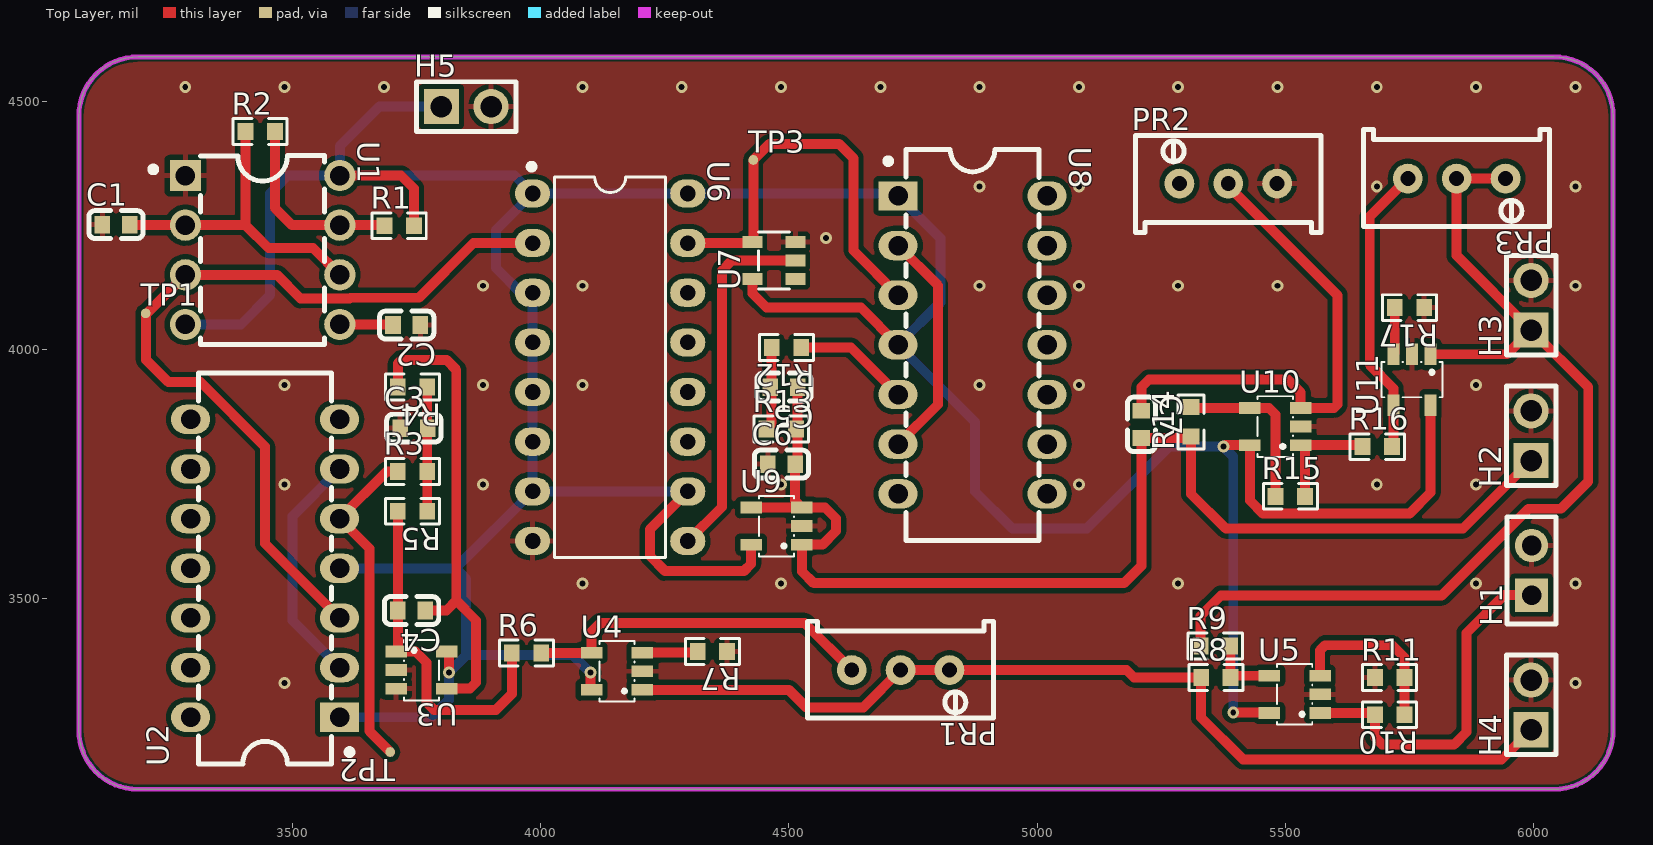
[diagram p0: Top Layer view]
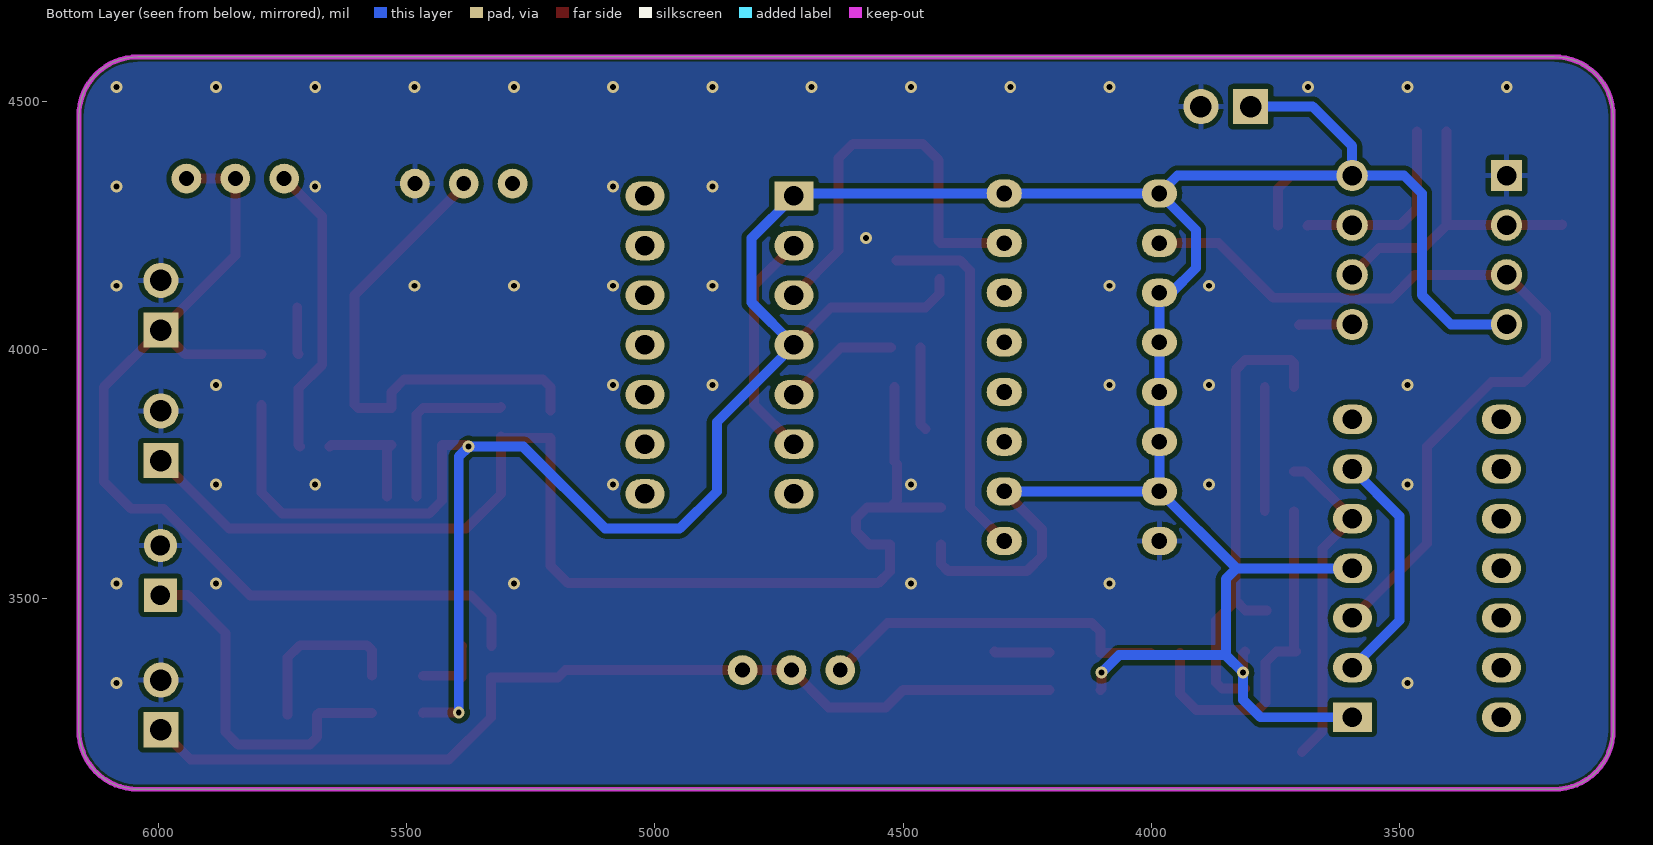
[diagram p1: Bottom Layer view, seen from below]
# Altium PCB MISC51901.pcbdoc
Units mil, origin at the board's own origin, x right, y up, seen from the top; angles counter-clockwise.
Board outline 3090 x 1475 mil, 2 copper layers (Top Layer, Bottom Layer), stack 62.206 mil thick; 46 components, 29 nets, 157 pads, 49 vias.

## Layer stack, top to bottom
Top Solder Mask Layer: solder mask 0.394, Dk 3.3
Top Layer: signal copper 1.379
Dielectric1: surface 59.449, FR4, Dk 4.5
Bottom Layer: signal copper 1.378
Bottom Solder Mask Layer: solder mask 0.394, Dk 3.3

## Board outline
3188.11,4590 ccw(c3188.11,4471.89) 3070,4471.89 3070,3233.11 ccw(c3188.11,3233.11) 3188.11,3115 6041.89,3115 ccw(c6041.89,3233.11) 6160,3233.11 6160,4471.89 ccw(c6041.89,4471.89) 6041.89,4590

## Design rules (kind name [scope] priority, off if disabled: settings)
BoardOutlineClearance copperThickness2oz_1 [All] p2 off: genericclearance=7.99 ignorepadtopadclearanceinfootprint=FALSE except(0: Arc-SplitContinuation Track-SplitContinuation SMDPad-SplitContinuation THPad-SplitContinuation Via-SplitContinuation Fill-SplitContinuation Region-SplitContinuation Poly-SplitContinuation Text-SplitContinuation Hole-SplitContinuation; 5.98: Arc-CutoutEdge Track-CutoutEdge SMDPad-CutoutEdge THPad-CutoutEdge Via-CutoutEdge Text-CutoutEdge; 6.9: Hole-OutlineEdge Hole-CutoutEdge; 10: Poly-OutlineEdge Poly-CutoutEdge; 11.81: Arc-OutlineEdge Track-OutlineEdge SMDPad-OutlineEdge THPad-OutlineEdge Via-OutlineEdge Fill-OutlineEdge Region-OutlineEdge Text-OutlineEdge Fill-CutoutEdge Region-CutoutEdge)
BoardOutlineClearance Plane_innerPlane_1 [All] p4 off: genericclearance=4.02 ignorepadtopadclearanceinfootprint=FALSE except(0: Arc-SplitContinuation Track-SplitContinuation SMDPad-SplitContinuation THPad-SplitContinuation Via-SplitContinuation Fill-SplitContinuation Region-SplitContinuation Poly-SplitContinuation Text-SplitContinuation Hole-SplitContinuation; 5.98: Arc-CutoutEdge Track-CutoutEdge SMDPad-CutoutEdge THPad-CutoutEdge Via-CutoutEdge Text-CutoutEdge; 6.9: Hole-OutlineEdge Hole-CutoutEdge; 10: Poly-OutlineEdge Poly-CutoutEdge; 11.81: Arc-OutlineEdge Track-OutlineEdge SMDPad-OutlineEdge THPad-OutlineEdge Via-OutlineEdge Fill-OutlineEdge Region-OutlineEdge Text-OutlineEdge Fill-CutoutEdge Region-CutoutEdge)
BoardOutlineClearance Copper_copperRegion_1 [All] p6 off: genericclearance=4.02 ignorepadtopadclearanceinfootprint=FALSE except(0: Arc-SplitContinuation Track-SplitContinuation SMDPad-SplitContinuation THPad-SplitContinuation Via-SplitContinuation Fill-SplitContinuation Region-SplitContinuation Poly-SplitContinuation Text-SplitContinuation Hole-SplitContinuation; 5.98: Arc-CutoutEdge Track-CutoutEdge SMDPad-CutoutEdge THPad-CutoutEdge Via-CutoutEdge Text-CutoutEdge; 6.9: Hole-OutlineEdge Hole-CutoutEdge; 10: Poly-OutlineEdge Poly-CutoutEdge; 11.81: Arc-OutlineEdge Track-OutlineEdge SMDPad-OutlineEdge THPad-OutlineEdge Via-OutlineEdge Fill-OutlineEdge Region-OutlineEdge Text-OutlineEdge Fill-CutoutEdge Region-CutoutEdge)
BoardOutlineClearance copperThickness1oz_1 [All] p8: genericclearance=4.02 ignorepadtopadclearanceinfootprint=FALSE except(0: Arc-SplitContinuation Track-SplitContinuation SMDPad-SplitContinuation THPad-SplitContinuation Via-SplitContinuation Fill-SplitContinuation Region-SplitContinuation Poly-SplitContinuation Text-SplitContinuation Hole-SplitContinuation; 5.98: Arc-CutoutEdge Track-CutoutEdge SMDPad-CutoutEdge THPad-CutoutEdge Via-CutoutEdge Text-CutoutEdge; 6.9: Hole-OutlineEdge Hole-CutoutEdge; 10: Poly-OutlineEdge Poly-CutoutEdge; 11.81: Arc-OutlineEdge Track-OutlineEdge SMDPad-OutlineEdge THPad-OutlineEdge Via-OutlineEdge Fill-OutlineEdge Region-OutlineEdge Text-OutlineEdge Fill-CutoutEdge Region-CutoutEdge)
Clearance copperThickness2oz [All] p1 off: gap=7.99 ignorepadtopadclearanceinfootprint=FALSE except(5.98: SMDPad-Track SMDPad-SMDPad THPad-Track SMDPad-THPad THPad-THPad Track-Via SMDPad-Via THPad-Via Via-Via Fill-SMDPad Region-SMDPad Fill-THPad Region-THPad Fill-Via Region-Via Fill-Fill Fill-Region Region-Region Arc-Track Arc-SMDPad Arc-THPad Arc-Via Fill-Arc Region-Arc Arc-Arc Text-Track SMDPad-Text Text-THPad Text-Via Fill-Text Region-Text Arc-Text Text-Text; 6.9: Hole-Track Hole-SMDPad Hole-THPad Hole-Via Fill-Hole Region-Hole Hole-Arc Hole-Text; 10: Poly-Track Poly-SMDPad Poly-THPad Poly-Via Poly-Fill Poly-Region Poly-Poly Poly-Arc Poly-Text Poly-Hole; 11.81: Fill-Track Region-Track)
Clearance Plane_innerPlane [All] p3 off: gap=4.02 ignorepadtopadclearanceinfootprint=FALSE except(5.98: SMDPad-Track SMDPad-SMDPad THPad-Track SMDPad-THPad THPad-THPad Track-Via SMDPad-Via THPad-Via Via-Via Fill-SMDPad Region-SMDPad Fill-THPad Region-THPad Fill-Via Region-Via Fill-Fill Fill-Region Region-Region Arc-Track Arc-SMDPad Arc-THPad Arc-Via Fill-Arc Region-Arc Arc-Arc Text-Track SMDPad-Text Text-THPad Text-Via Fill-Text Region-Text Arc-Text Text-Text; 6.9: Hole-Track Hole-SMDPad Hole-THPad Hole-Via Fill-Hole Region-Hole Hole-Arc Hole-Text; 10: Poly-Track Poly-SMDPad Poly-THPad Poly-Via Poly-Fill Poly-Region Poly-Poly Poly-Arc Poly-Text Poly-Hole; 11.81: Fill-Track Region-Track)
Clearance Copper_copperRegion [All] p5 off: gap=4.02 ignorepadtopadclearanceinfootprint=FALSE except(5.98: SMDPad-Track SMDPad-SMDPad THPad-Track SMDPad-THPad THPad-THPad Track-Via SMDPad-Via THPad-Via Via-Via Fill-SMDPad Region-SMDPad Fill-THPad Region-THPad Fill-Via Region-Via Fill-Fill Fill-Region Region-Region Arc-Track Arc-SMDPad Arc-THPad Arc-Via Fill-Arc Region-Arc Arc-Arc Text-Track SMDPad-Text Text-THPad Text-Via Fill-Text Region-Text Arc-Text Text-Text; 6.9: Hole-Track Hole-SMDPad Hole-THPad Hole-Via Fill-Hole Region-Hole Hole-Arc Hole-Text; 10: Poly-Track Poly-SMDPad Poly-THPad Poly-Via Poly-Fill Poly-Region Poly-Poly Poly-Arc Poly-Text Poly-Hole; 11.81: Fill-Track Region-Track)
Clearance copperThickness1oz [All] p7: gap=4.02 ignorepadtopadclearanceinfootprint=FALSE except(5.98: SMDPad-Track SMDPad-SMDPad THPad-Track SMDPad-THPad THPad-THPad Track-Via SMDPad-Via THPad-Via Via-Via Fill-SMDPad Region-SMDPad Fill-THPad Region-THPad Fill-Via Region-Via Fill-Fill Fill-Region Region-Region Arc-Track Arc-SMDPad Arc-THPad Arc-Via Fill-Arc Region-Arc Arc-Arc Text-Track SMDPad-Text Text-THPad Text-Via Fill-Text Region-Text Arc-Text Text-Text; 6.9: Hole-Track Hole-SMDPad Hole-THPad Hole-Via Fill-Hole Region-Hole Hole-Arc Hole-Text; 10: Poly-Track Poly-SMDPad Poly-THPad Poly-Via Poly-Fill Poly-Region Poly-Poly Poly-Arc Poly-Text Poly-Hole; 11.81: Fill-Track Region-Track)
DiffPairsRouting differentialPair [All] p1: maxlimit=6 minlimit=6 mostfreqgap=6 toplayer_minwidth=5 toplayer_prefwidth=10 toplayer_maxwidth=100 toplayer_mingap=6 toplayer_prefgap=6 toplayer_maxgap=6 bottomlayer_minwidth=5 bottomlayer_prefwidth=10 bottomlayer_maxwidth=100 bottomlayer_mingap=6 bottomlayer_prefgap=6 bottomlayer_maxgap=6 maxuncoupledlength=10
HoleToHoleClearance otherClearance [All] p1: gap=11.81 allowstackedmicrovias=TRUE
Length netLength [All] p1: minlimit=0 maxlimit=0
PasteMaskExpansion pasteMaskExpansion [All] p1: expansion=0
PlaneConnect innerPlane [All] p1: planeconnectstyle=Relief reliefexpansion=20 reliefentries=4 reliefconductorwidth=10 reliefairgap=10
PolygonConnect copperRegion [All] p1: connectstyle=Relief reliefconductorwidth=10 reliefentries=4 polygonreliefangle="90 Angle" airgapwidth=10 via.connectstyle=Relief via.reliefconductorwidth=10 via.reliefentries=4 via.polygonreliefangle="90 Angle" via.airgapwidth=10
RoutingVias viaSize [All] p1: holewidth=12.01 width=24.02 viastyle="Through Hole" minholewidth=11.81 minwidth=19.68 maxholewidth=248.03 maxwidth=393.7
SolderMaskExpansion solderMaskExpansion [IsVia] p1: expansion=-1000 istentingtop=TRUE
SolderMaskExpansion solderMaskExpansion [All] p2: expansion=2 istentingtop=FALSE
Width copperThickness2oz_2 [All] p1 off: maxlimit=100 minlimit=8 preferedwidth=10
Width copperThickness1oz_2 [All] p2: maxlimit=100 minlimit=5 preferedwidth=10

## Components (designator, comment, footprint, x,y, rotation, side; value= is the part's Value field where it differs from the comment)
C1 "5nF" C0603 3144.72,4252.4 r0 top
C2 "0.22uF" C0603 3730,4050 r180 top
C3 "5.1nF" C0603 3744.64,3842.36 r0 top
C4 "1nF" C0603 3740,3475 r180 top
C5 "3300pF" C0603 4490,3925 r180 top
C6 "3300pF" C0603 4485,3770 r0 top
C7 "1nF" C0603 5210,3850 r270 top
H1 "" HDR-TH_2P-P2.54-V-F 5995.79,3555.96 r90 top
H2 "" HDR-TH_2P-P2.54-V-M-1 5995,3826.92 r90 top
H3 "" HDR-TH_2P-P2.54-V-M-1 5995,4090 r90 top
H4 "" HDR-TH_2P-P2.54-V-M-1 5995,3285 r90 top
H5 "" HDR-TH_2P-P2.54-V-M-1 3850,4490 r0 top
PR1 "10kΩ" R_3296 4725,3350 r180 top
PR2 "10kΩ" R_3296 5385,4340 r0 top
PR3 "10kΩ" R_3296 5845,4340 r180 top
R1 "1.2K" R0603 3715,4250 r0 top
R2 "1.8K" R0603 3435,4440 r0 top
R3 "2K" R0603 3741.91,3754.99 r0 top
R4 "2K" R0603 3741.91,3924.99 r180 top
R5 "2.7K" R0603 3741.91,3674.99 r180 top
R6 "2K" R0603 3971.55,3389.32 r0 top
R7 "2K" R0603 4345.87,3392.64 r180 top
R8 "10K" R0603 5360,3340 r0 top
R9 "10K" R0603 5358.63,3403.66 r0 top
R10 "10K" R0603 5710,3265 r180 top
R11 "10K" R0603 5710,3340 r0 top
R12 "5.1K" R0603 4495,4005 r180 top
R13 "5.1K" R0603 4484.61,3840.51 r0 top
R14 "10K" R0603 5310,3855 r90 top
R15 "10K" R0603 5510,3705 r0 top
R16 "2K" R0603 5685,3805 r0 top
R17 "2K" R0603 5750,4085 r180 top
TP1 "" Test-Point-0.5mm 3204.49,4073.66 r0 top
TP2 "" Test-Point-0.5mm 3696.91,3189.99 r180 top
TP3 "" Test-Point-0.5mm 4428.26,4382.6 r0 top
U1 "NE555" PDIP-8_L9.6-W6.4-P2.54-LS7.9-BL-1 3439.97,4201.14 r270 top
U2 "DM7474N" PDIP-14_L19.5-W6.7-P2.54-LS7.9-BL 3445,3560 r90 top
U3 "OPAMP_3T_VIRTUAL" SOT-23-5_L3.0-W1.7-P0.95-LS2.8-BR 3760,3355 r180 top
U4 "OPAMP_3T_VIRTUAL" SOT-23-5_L3.0-W1.7-P0.95-LS2.8-BR 4153.63,3352.64 r0 top
U5 "OPAMP_3T_VIRTUAL" SOT-23-5_L3.0-W1.7-P0.95-LS2.8-BR 5518.68,3306.14 r0 top
U6 "74LS161N" PDIP-16_L19.3-W6.4-P2.54-LS7.94-BL 4140,3965 r270 top
U7 "HSN74LVC1G04DBVR" SOT-23-5_L2.9-W1.6-P0.95-LS2.9-BL 4470,4180 r90 top
U8 "DM7474N" PDIP-14_L19.5-W6.7-P2.54-LS7.9-BL 4870,4010 r270 top
U9 "OPAMP_3T_VIRTUAL" SOT-23-5_L3.0-W1.7-P0.95-LS2.8-BR 4475,3645 r0 top
U10 "OPAMP_3T_VIRTUAL" SOT-23-5_L3.0-W1.7-P0.95-LS2.8-BR 5479.6,3845.51 r0 top
U11 "OPAMP_3T_VIRTUAL" SOT-23-5_L3.0-W1.7-P0.95-LS2.8-BR 5755,3940 r90 top

## Footprints (in the part's own frame and the unit in brackets; to place one, negate y for a bottom-side part, rotate by r counter-clockwise, add the part's x,y. Pads: shape width x height; smd on the part's side, far side on the other; paste and mask are expansions set on the pad)
C0603 [mm]
  rect 0.8x0.9 smd: 1(-0.7,0) 2(0.7,0)
  silkscreen extent -1.39,-0.71 1.39,0.71
HDR-TH_2P-P2.54-V-F [mm]
  rect 1.7x1.7 hole 1: 1(-1.27,0)
  round 1.7 hole 1: 2(1.27,0)
  silkscreen extent -2.74,-1.25 2.74,1.25
HDR-TH_2P-P2.54-V-M-1 [mm]
  rect 1.8x1.8 hole 1.1: 1(-1.27,0)
  round 1.8 hole 1.1: 2(1.27,0)
  silkscreen extent -2.54,-1.27 2.54,1.27
PDIP-8_L9.6-W6.4-P2.54-LS7.9-BL-1 [mil]
  rect 63x63 hole 39.37: 1(-150,-155.51)
  round 63 hole 39.37: 2(-50,-155.51) 3(50,-155.51) 4(150,-155.51) 5(150,155.52) 6(50,155.52) 7(-50,155.52) 8(-150,155.52)
  silkscreen extent -190,-226 190,125
PDIP-14_L19.5-W6.7-P2.54-LS7.9-BL [mm]
  rect 1.5x2 hole 1: 1(-7.62,-3.81)
  oval 1.5x2 hole 1: 2(-5.08,-3.81) 3(-2.54,-3.81) 4(0,-3.81) 5(2.54,-3.81) 6(5.08,-3.81) 7(7.62,-3.81)
  oval 1.5x2 hole 1 copper offset 0,0: 8(7.62,3.81) 9(5.08,3.81) 10(2.54,3.81) 11(0,3.81) 12(-2.54,3.81) 13(-5.08,3.81) 14(-7.62,3.81)
  silkscreen extent -10,-4.47 10,3.4
PDIP-16_L19.3-W6.4-P2.54-LS7.94-BL [mm]
  oval 1.44x1.8 hole 0.8: 1(-8.89,-3.97) 2(-6.35,-3.97) 3(-3.81,-3.97) 4(-1.27,-3.97) 5(1.27,-3.97) 6(3.81,-3.97) 7(6.35,-3.97) 8(8.89,-3.97) 9(8.89,3.97) 10(6.35,3.97) 11(3.81,3.97) 12(1.27,3.97) 13(-1.27,3.97) 14(-3.81,3.97) 15(-6.35,3.97) 16(-8.89,3.97)
  silkscreen extent -10.41,-4.17 9.73,2.84
R0603 [mil]
  rect 31.75x34.02 smd paste-3937.01 mask+2: 1(-29.66,0) 2(29.66,0)
  silkscreen extent -55,-26 55,26
R_3296 [mil]
  round 60 hole 30 paste+0 mask+2: 1(-98.4,-5) 2(0,-5) 3(98.4,-5)
  silkscreen extent -187,-103 187,92
SOT-23-5_L2.9-W1.6-P0.95-LS2.9-BL [mm]
  rect 0.6x1 smd paste+0 mask+0.05: 1(-0.95,-1.1) 2(0,-1.1) 3(0.95,-1.1) 4(0.95,1.1) 5(-0.95,1.1)
  silkscreen extent -1.45,-0.8 1.45,0.8
SOT-23-5_L3.0-W1.7-P0.95-LS2.8-BR [mm]
  rect 1.1x0.6 smd: 1(1.3,-0.95) 2(1.3,0) 3(1.3,0.95) 4(-1.3,0.95) 5(-1.3,-0.95)
  silkscreen extent -0.9,-1.55 0.9,1.55
Test-Point-0.5mm [mm]
  round 0.5 smd: 1(0,0)

## Via types
v1: diameter 24.02, hole 12, Top Layer to Bottom Layer, 45 vias
v2: diameter 24, hole 12, Top Layer to Bottom Layer, 4 vias

## Nets (pads, with @x,y where several pads share a name; then routed paths per layer and width w, separated by ;. In a path a pad name is that pad's centre, name@x,y a point inside that pad or via, vN(x,y) a via of type N, cw(c..) or ccw(c..) an arc to the next point about the centre after c; other vN are vias at no path point)
$1N343: R1.1 R2.2 U1.7 | length 390
  Top Layer w20: R2.2 3464.66,4285.34 3498.86,4251.14 U1.7 3684.2,4251.14 R1.1
$1N384: C1.2 R2.1 U1.2 U1.6 | length 654
  Top Layer w20: C1.2 3173.54,4251.14 U1.2 3405.34,4251.14 ; R2.1 3405.34,4251.14 ; U1.6 3541.62,4205 3451.48,4205 3405.34,4251.14
$1N523: C2.2 U1.5 | length 107.4
  Top Layer w20: U1.5 3701.3,4051.14 C2.2
$1N540: TP1.1 U1.3 U2.3 U6.2 | length 1688.7
  Top Layer w20: U2.3 3445,3610 3445,3805 3315,3935 3250,3935 3205,3980 3205,4071.69 U1.3 3468.86,4151.14 3516.34,4103.66 3615.14,4103.66 3616.48,4105 3755,4105 3865,4215 U6.2
$1N1056: U2.2 U2.6 | length 478.7
  Bottom Layer w20: U2.2 3500,3455 3500,3665 U2.6
$1N1185: R3.1 TP2.1 U2.5 | length 668.8
  Top Layer w20: TP2.1 3655,3231.9 3655,3600 U2.5 3689.99,3754.99 R3.1
$1N1274: C4.1 R4.2 U3.4 | length 957.7
  Top Layer w20: R4.2 3712.24,3972.24 3720,3980 3810,3980 3830,3960 3830,3495 ; C4.1 3810,3475 3830,3495 ; U3.4 3857.6,3317.6 3870,3330 3870,3455 3830,3495
$1N1551: C3.2 R3.2 R4.1 R5.1 | length 250
  Top Layer w20: R5.1 R3.2 R4.1
$1N1752: C4.2 R5.2 R6.1 U3.1 | length 708.2
  Top Layer w20: R5.2 3712.24,3395.83 U3.1 3747.6,3392.4 3770,3370 3770,3290 3785,3275 3910,3275 3941.89,3306.89 R6.1
$1N1828: H4.1 PR1.1 PR1.2 R8.1 U4.1 | length 1982.3
  Top Layer w20: U4.1 4499.76,3315.24 4535,3280 4650,3280 PR1.2 PR1.1 5180,3355 5195,3340 R8.1 5330.34,3259.66 5415,3175 5935,3175 H4.1
$1N1834: PR1.3 R6.2 U4.4 | length 714.7
  Top Layer w20: R6.2 4101.73,3389.32 U4.4 4102.44,3432.45 4120,3450 4531.6,3450 PR1.3
$1N1887: R7.2 U4.3 | length 112.5
  Top Layer w20: U4.3 4313.61,3390.04 R7.2
$1N2098: R8.2 R9.2 U5.4 | length 143.5
  Top Layer w20: R9.2 5389.66,3402.29 R8.2 5393.2,3343.54 U5.4
$1N2118: R10.1 R11.2 U5.3 | length 350.9
  Top Layer w20: U5.3 5569.87,3394.87 5580,3405 5715,3405 5739.66,3380.34 R11.2 R10.1
$1N2145: H1.1 R10.2 U5.1 | length 720.7
  Top Layer w20: U5.1 5676.6,3268.74 R10.2 5680.34,3219.66 5695,3205 5840,3205 5865,3230 5865,3430 5940.96,3505.96 H1.1
$1N3520: U6.9 U7.2 | length 730.1
  Top Layer w20: U6.9 4365,3683.7 4365,4160 4385,4180 U7.2
$1N3951: C5.2 R12.2 R13.1 | length 168.8
  Top Layer w20: R13.1 4465.34,3850.89 R12.2
$1N3954: R12.1 U8.5 | length 234.7
  Top Layer w20: R12.1 4625,4005 U8.5
$1N4573: R14.2 R15.1 U10.4 | length 341.2
  Top Layer w20: R14.2 5311.75,3882.91 U10.4 5467.09,3882.91 5480,3870 5480,3705.34 R15.1
$1N4623: C7.1 PR2.2 U10.3 | length 1029.7
  Top Layer w20: C7.1 5210,3925 5225,3940 5505,3940 5530.79,3914.21 U10.3 5597.91,3882.91 5605,3890 5605,4110 5385,4330 PR2.2
$1N4638: C5.1 C6.2 C7.2 H2.1 R13.2 R14.1 U9.1 U9.3 U9.4 | length 2542.6
  Top Layer w20: U9.4 U9.3 ; C5.1 4517.56,3775 C6.2 4512.56,3696.03 U9.3 ; H2.1 5858.08,3640 5380,3640 5310,3710 R14.1 5307.1,3822.44 C7.2 5210,3565 5175,3530 4550,3530 4526.19,3553.82 U9.1 4567.6,3607.6 4595,3635 4595,3660 4572.6,3682.4 U9.3
$1N4755: R15.2 R16.1 U10.1 | length 232.6
  Top Layer w20: R15.2 5539.66,3799.24 U10.1 5652.23,3808.11 R16.1
$1N4949: R17.2 U11.3 | length 94.9
  Top Layer w20: U11.3 5720.34,3993.93 R17.2
$1N5043: H3.1 PR3.1 PR3.2 R9.1 U11.1 | length 1994.6
  Top Layer w20: R9.1 5328.97,3463.97 5370,3505 5815,3505 5990,3680 6055,3680 6110,3735 6110,3925 H3.1 ; U11.1 5946.19,3991.18 H3.1 ; PR3.1 PR3.2 5845,4190 H3.1
$1N5049: PR3.3 R16.2 U11.4 | length 592.7
  Top Layer w20: R16.2 5717.6,3807.94 U11.4 5717.6,3922.4 5670,3970 5670,4268.4 PR3.3
$1N5276: U8.2 U8.6 | length 466.3
  Top Layer w20: U8.6 4800,3890 4800,4130 U8.2
$1N5285: TP3.1 U6.15 U7.4 U8.3 | length 837.6
  Top Layer w20: U6.15 4424.29,4215 U7.4 4428.26,4218.98 TP3.1 4460.67,4415 4600.89,4415 4630,4385.89 4630,4200 U8.3
GND: C1.1 C2.1 C3.1 C6.1 H1.2 H2.2 H3.2 H4.2 H5.2 PR2.3 R7.1 R11.1 R17.1 U1.1 U3.2 U3.3 U4.2 U5.2 U6.8 U7.3 U9.2 U10.2 U11.2
  other v1: 3484.1,3329.1 6084.1,3329.1 4084.1,3529.1 4484.1,3529.1 5284.1,3529.1 5884.1,3529.1 6084.1,3529.1 3484.1,3729.1 3884.1,3729.1 4484.1,3729.1 5084.1,3729.1 5684.1,3729.1 5884.1,3729.1 3484.1,3929.1 3884.1,3929.1 4084.1,3929.1 4884.1,3929.1 5084.1,3929.1 5884.1,3929.1 3884.1,4129.1 4084.1,4129.1 4884.1,4129.1 5084.1,4129.1 5284.1,4129.1 5484.1,4129.1 6084.1,4129.1 4575,4225 4884.1,4329.1 5084.1,4329.1 5684.1,4329.1 6084.1,4329.1 3284.1,4529.1 3484.1,4529.1 3684.1,4529.1 4084.1,4529.1 4284.1,4529.1 4484.1,4529.1 4684.1,4529.1 4884.1,4529.1 5084.1,4529.1 5284.1,4529.1 5484.1,4529.1 5684.1,4529.1 5884.1,4529.1 6084.1,4529.1
VCC: H5.1 R1.2 U1.4 U1.8 U2.1 U2.4 U3.5 U4.5 U5.5 U6.1 U6.3 U6.4 U6.5 U6.6 U6.7 U6.10 U6.16 U7.5 U8.1 U8.4 U9.5 U10.5 U11.5 | length 8004.8
  Top Layer w20: U1.8 3718.86,4351.14 3744.66,4325.34 R1.2 ; U3.5 3815,3388.59 v2(3815,3350) ; v2(4100,3350) 4100,3317.68 U4.5 ; U6.10 4220,3638.7 4220,3585 4250,3555 4410,3555 4423.81,3568.82 U9.5 ; U7.5 4426.69,4113.31 4455,4085 4645,4085 U8.4 ; v2(5375,3805) 5378.11,3808.11 U10.5 5428.42,3696.58 5455,3670 5750,3670 5792.4,3712.4 U11.5 ; v2(5395,3270) 5466.24,3270 U5.5
  Bottom Layer w20: U1.4 3396.14,4051.14 3455,4110 3455,4315 3491.14,4351.14 U1.8 ; U2.1 3780,3260 3815,3295 v2(3815,3350) 3850,3385 ; U2.4 3828.7,3560 ; H5.1 3675,4490 3595.47,4410.48 U1.8 ; v2(4100,3350) 4065,3385 3850,3385 ; U6.10 U6.7 ; v2(5395,3270) 5395,3785 v2(5375,3805) 5265,3805 5100,3640 4950,3640 4875,3715 4875,3855 U8.4 4805,4095 4805,4225.01 U8.1 4715.01,4315 U6.16 U6.1 ; U1.8 3947.56,4351.14 U6.1 ; 3828.7,3560 U6.7 ; 3828.7,3560 3850,3538.7 3850,3385 ; U6.7 U6.6 U6.5 U6.4 U6.3 3960,4115 3910,4165 3910,4241.3 U6.1
pads on no net: PR2.1 U2.7 U2.8 U2.9 U2.10 U2.11 U2.12 U2.13 U2.14 U6.11 U6.12 U6.13 U6.14 U7.1 U8.7 U8.8 U8.9 U8.10 U8.11 U8.12 U8.13 U8.14

## Polygon pours and split planes (outlines as drawn)
GND on Top Layer (solid, remove dead copper, pour order 0): 3010,4720 3010,3000 6310,3000 6310,4720
GND on Bottom Layer (solid, remove dead copper, pour order 2): 3000,4705 3000,3010 6295,3010 6295,4705

## Keep-outs
Board Outline Layer:
  the board outline again, w10